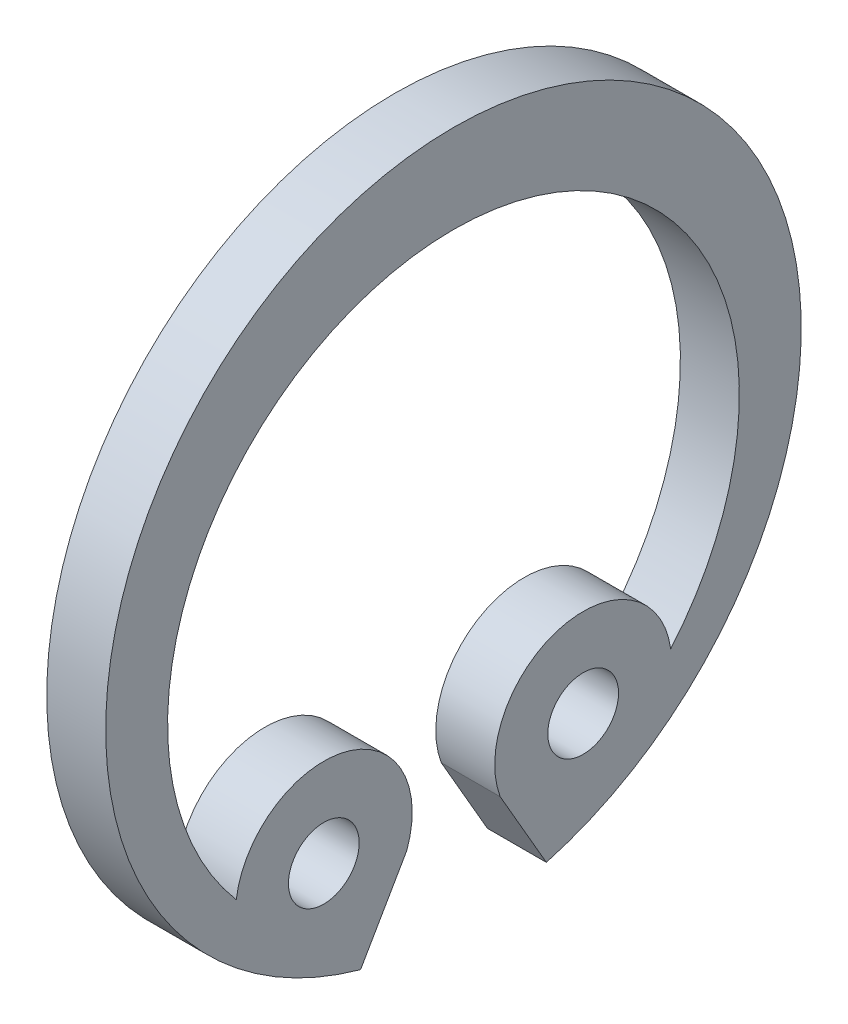
from build123d import *

# Parameters (mm, degrees)
EXTRUDE_1_DEPTH      = 0.5
EXTRUDE_1_DEPTH_BACK = 0.5
SKETCH_1_R           = 0.6


with BuildPart() as part:
    # 草图1 → 凸台-拉伸1 (new, two sides: drawn at the far end of the back side and taken through both)
    with BuildSketch(Plane(origin=(0, 0, 0), x_dir=(0, 0, -1), z_dir=(1, 0, 0)).offset(-EXTRUDE_1_DEPTH_BACK)):
        with BuildLine():
            Line((-1.575903864, -5.685642181), (-0.792131706, -4.328108982))
            ThreePointArc((-0.792131706, -4.328108982), (-1.835210176, -2.355544978), (-3.685531471, -3.602674702))
            ThreePointArc((-3.685531471, -3.602674702), (0, 4.4), (3.685531471, -3.602674702))
            ThreePointArc((3.685531471, -3.602674702), (1.835210176, -2.355544978), (0.792131706, -4.328108982))
            Line((0.792131706, -4.328108982), (1.575903864, -5.685642181))
            ThreePointArc((1.575903864, -5.685642181), (0, 5.9), (-1.575903864, -5.685642181))
        make_face()
        with Locations((2.2, -3.810511777)):
            Circle(SKETCH_1_R, mode=Mode.SUBTRACT)
        with Locations((-2.2, -3.810511777)):
            Circle(SKETCH_1_R, mode=Mode.SUBTRACT)
    extrude(amount=EXTRUDE_1_DEPTH + EXTRUDE_1_DEPTH_BACK)


solid = part.part
